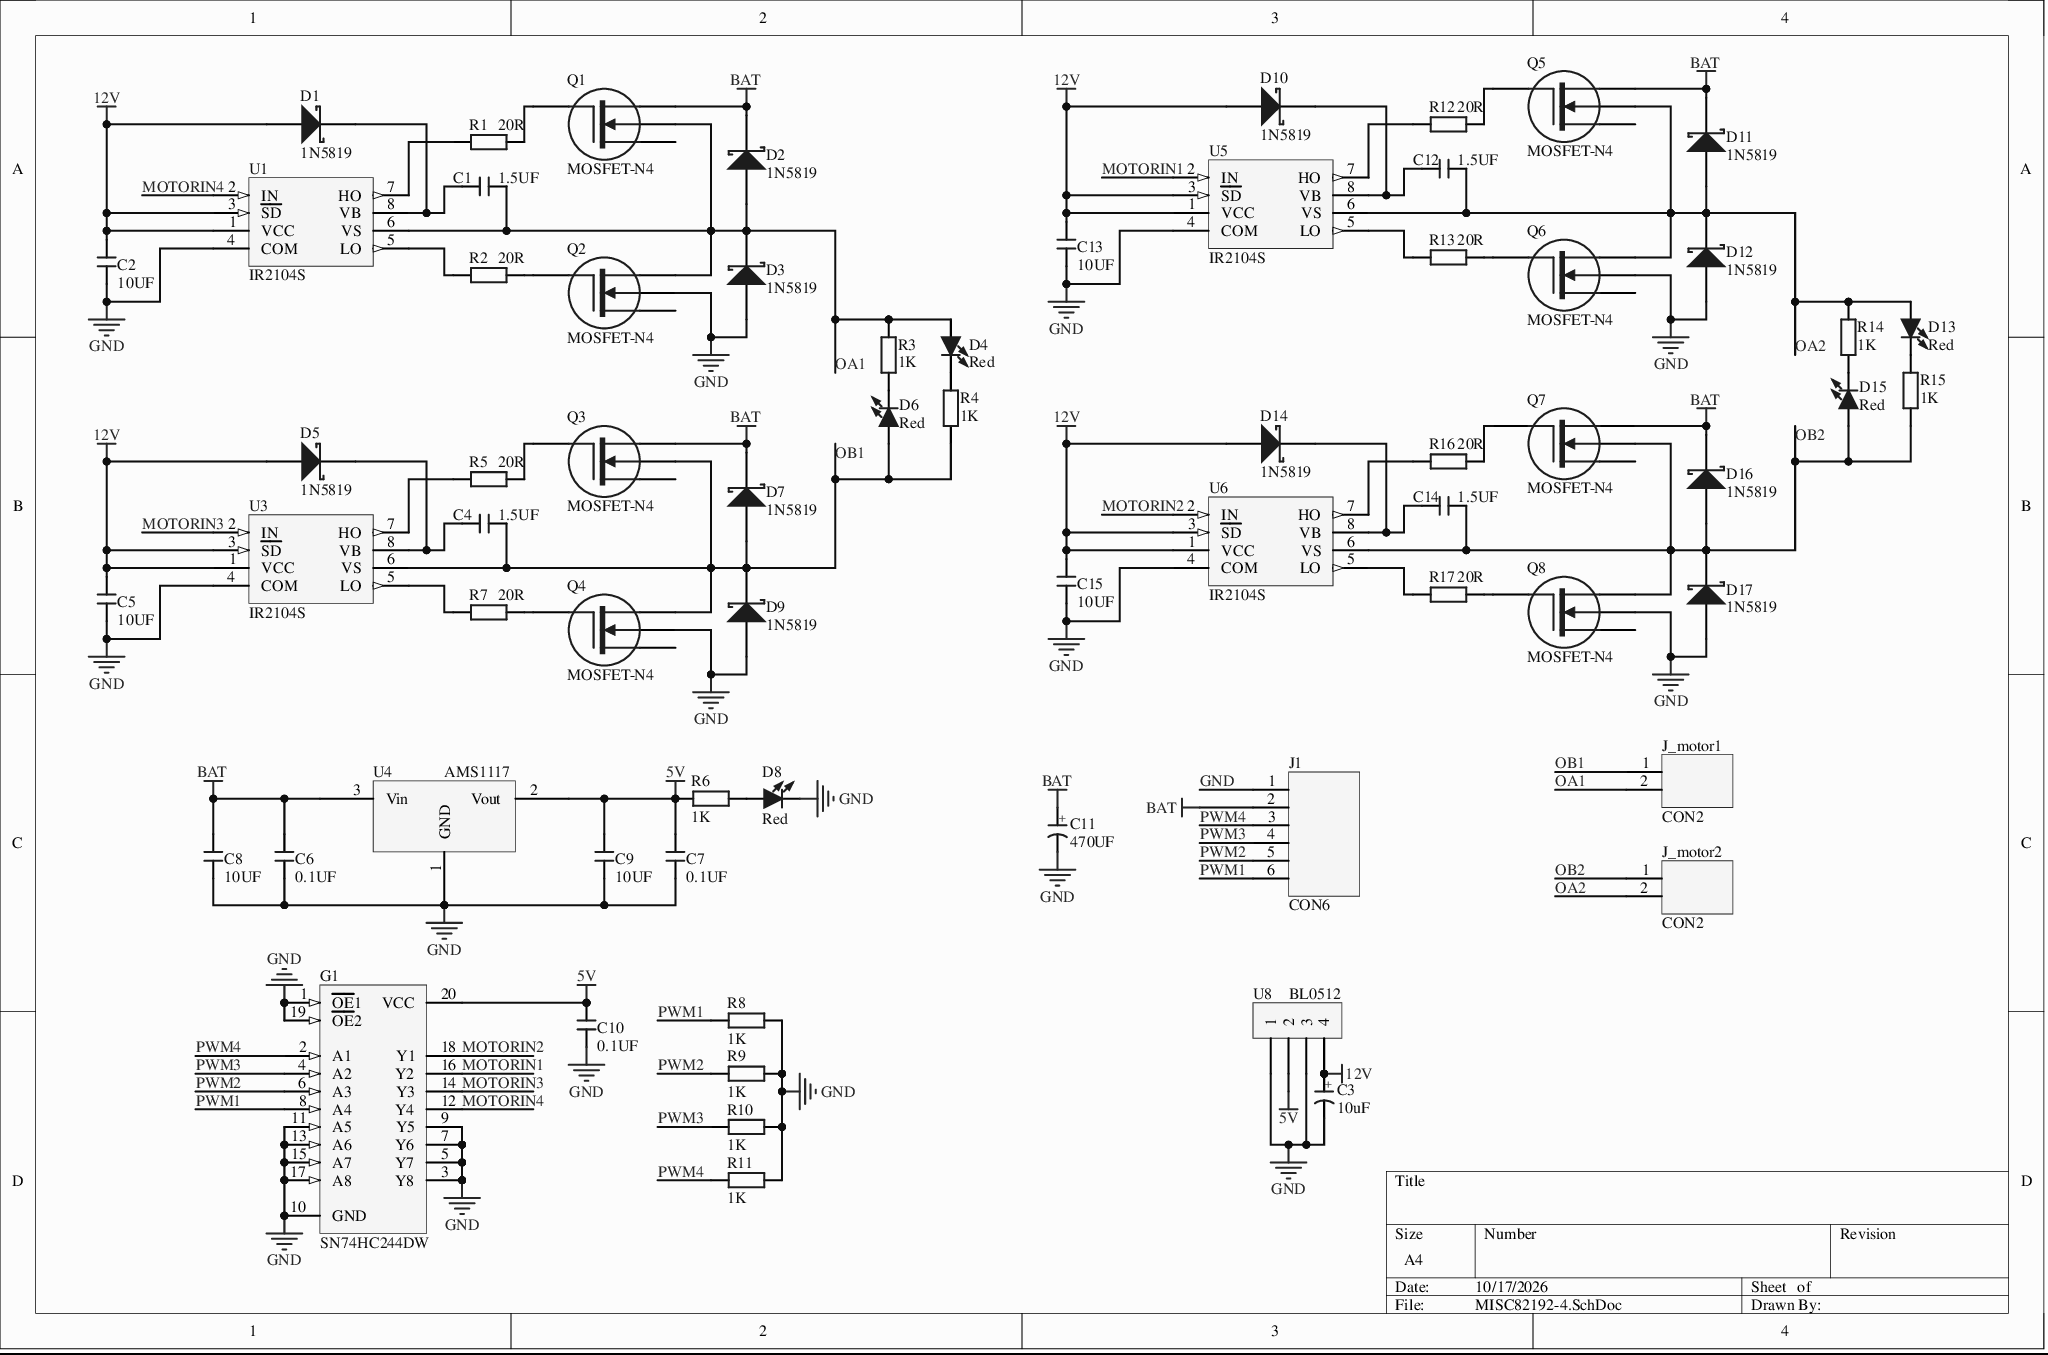
[diagram p0: MISC82192-4.SchDoc]
# Altium project MISC82192-7.PrjPcb
1 sheet, 67 parts. Net scope: global (net labels, ports and power ports of the same name join across sheets).
Board file: MISC82192.PcbDoc

## Sheet MISC82192-4.SchDoc
size A4

### Parts
C1  1.5UF  [C 0805_L]
C2  10UF  [C 0805_L]
C3  10uF  [C 0805_L]
C4  1.5UF  [C 0805_L]
C5  10UF  [C 0805_L]
C6  0.1UF  [C 0805_L]
C7  0.1UF  [C 0805_L]
C8  10UF  [C 0805_L]
C9  10UF  [C 0805_L]
C10  0.1UF  [C 0805_L]
C11  470UF  [CM A(3*5.4)]
C12  1.5UF  [C 0805_L]
C13  10UF  [C 0805_L]
C14  1.5UF  [C 0805_L]
C15  10UF  [C 0805_L]
D1  1N5819  [SOD-323]
D2  1N5819  [SOD-323]
D3  1N5819  [SOD-323]
D4  Red  [LED 0805G]
D5  1N5819  [SOD-323]
D6  Red  [LED 0805G]
D7  1N5819  [SOD-323]
D8  Red  [LED 0805G]
D9  1N5819  [SOD-323]
D10  1N5819  [SOD-323]
D11  1N5819  [SOD-323]
D12  1N5819  [SOD-323]
D13  Red  [LED 0805G]
D14  1N5819  [SOD-323]
D15  Red  [LED 0805G]
D16  1N5819  [SOD-323]
D17  1N5819  [SOD-323]
G1  SN74HC244DW  [DW020]
J1  CON6  [PH2.0-6P]
J_motor1  CON2  [PH2.0-2P]
J_motor2  CON2  [PH2.0-2P]
Q1  MOSFET-N4  [TO252]
Q2  MOSFET-N4  [TO252]
Q3  MOSFET-N4  [TO252]
Q4  MOSFET-N4  [TO252]
Q5  MOSFET-N4  [TO252]
Q6  MOSFET-N4  [TO252]
Q7  MOSFET-N4  [TO252]
Q8  MOSFET-N4  [TO252]
R1  20R  [R 0805_L]
R2  20R  [R 0805_L]
R3  1K  [R 0805_L]
R4  1K  [R 0805_L]
R5  20R  [R 0805_L]
R6  1K  [R 0805_L]
R7  20R  [R 0805_L]
R8  1K  [R 0805_L]
R9  1K  [R 0805_L]
R10  1K  [R 0805_L]
R11  1K  [R 0805_L]
R12  20R  [R 0805_L]
R13  20R  [R 0805_L]
R14  1K  [R 0805_L]
R15  1K  [R 0805_L]
R16  20R  [R 0805_L]
R17  20R  [R 0805_L]
U1  IR2104S  [SOP8]
U3  IR2104S  [SOP8]
U4  AMS1117  [SOT223]
U5  IR2104S  [SOP8]
U6  IR2104S  [SOP8]
U8  BL0512  [Fe-HDR1X4/2.54-S]

### Nets
5V: C7.2 C9.2 C10.2 G1.20(VCC) R6.1 U4.2(Vout) U8.2
12V: C2.2 C3.1(A) C5.2 C13.2 C15.2 D1.1(A) D5.1(A) D10.1(A) D14.1(A) U1.1(VCC) U1.3(~{SD}) U3.1(VCC) U3.3(~{SD}) U5.1(VCC) U5.3(~{SD}) U6.1(VCC) U6.3(~{SD}) U8.4
BAT: C6.2 C8.2 C11.1(A) D2.2(K) D7.2(K) D11.2(K) D16.2(K) J1.2 Q1.4(S) Q3.4(S) Q5.4(S) Q7.4(S) U4.3(Vin)
GND: C2.1 C3.2(K) C5.1 C6.1 C7.1 C8.1 C9.1 C10.1 C11.2(K) C13.1 C15.1 D3.1(A) D8.2(K) D9.1(A) D12.1(A) D17.1(A) G1.1(~{OE}1) G1.3(Y8) G1.5(Y7) G1.7(Y6) G1.9(Y5) G1.10(GND) G1.11(A5) G1.13(A6) G1.15(A7) G1.17(A8) G1.19(~{OE}2) J1.1 Q2.3(U) Q4.3(U) Q6.3(U) Q8.3(U) R8.2 R9.2 R10.2 R11.2 U1.4(COM) U3.4(COM) U4.1(GND) U5.4(COM) U6.4(COM) U8.1 U8.3
MOTORIN1: G1.16(Y2) U5.2(IN)
MOTORIN2: G1.18(Y1) U6.2(IN)
MOTORIN3: G1.14(Y3) U3.2(IN)
MOTORIN4: G1.12(Y4) U1.2(IN)
OA1: C1.1 D2.1(A) D3.2(K) D4.1(A) J_motor1.2 Q1.3(U) Q2.4(S) R3.2 U1.6(VS)
OA2: C12.1 D11.1(A) D12.2(K) D13.1(A) J_motor2.2 Q5.3(U) Q6.4(S) R14.2 U5.6(VS)
OB1: C4.1 D6.1(A) D7.1(A) D9.2(K) J_motor1.1 Q3.3(U) Q4.4(S) R4.2 U3.6(VS)
OB2: C14.1 D15.1(A) D16.1(A) D17.2(K) J_motor2.1 Q7.3(U) Q8.4(S) R15.2 U6.6(VS)
PWM1: G1.8(A4) J1.6 R8.1
PWM2: G1.6(A3) J1.5 R9.1
PWM3: G1.4(A2) J1.4 R10.1
PWM4: G1.2(A1) J1.3 R11.1
NetC1_2: C1.2 D1.2(K) U1.8(VB)
NetC4_2: C4.2 D5.2(K) U3.8(VB)
NetC12_2: C12.2 D10.2(K) U5.8(VB)
NetC14_2: C14.2 D14.2(K) U6.8(VB)
NetD4_2: D4.2(K) R4.1
NetD6_2: D6.2(K) R3.1
NetD8_1: D8.1(A) R6.2
NetD13_2: D13.2(K) R15.1
NetD15_2: D15.2(K) R14.1
NetQ1_1: Q1.1(G) R1.2
NetQ2_1: Q2.1(G) R2.2
NetQ3_1: Q3.1(G) R5.2
NetQ4_1: Q4.1(G) R7.2
NetQ5_1: Q5.1(G) R12.2
NetQ6_1: Q6.1(G) R13.2
NetQ7_1: Q7.1(G) R16.2
NetQ8_1: Q8.1(G) R17.2
NetR1_1: R1.1 U1.7(HO)
NetR2_1: R2.1 U1.5(LO)
NetR5_1: R5.1 U3.7(HO)
NetR7_1: R7.1 U3.5(LO)
NetR12_1: R12.1 U5.7(HO)
NetR13_1: R13.1 U5.5(LO)
NetR16_1: R16.1 U6.7(HO)
NetR17_1: R17.1 U6.5(LO)

Not connected (* = marked no-connect by the designer): Q1 2(D); Q2 2(D); Q3 2(D); Q4 2(D); Q5 2(D); Q6 2(D); Q7 2(D); Q8 2(D)

### Library data of the parts
C1 C2 C4-C10 C12-C15 = C: SMD capacitor; BOM名称: Non-polarized SMD capacitor
C3 = CS_SMD: SMD solid-state capacitor; BOM名称: SMD solid-state capacitor
C11 = CE_SMD: SMD electrolytic capacitor; BOM名称: SMD electrolytic capacitor
D1-D3 D5 D7 D9-D12 D14 D16 D17 = 1N5819: Schottky diode; 属性: 40V/2A; BOM名称: Schottky diode
D4 D6 D8 D13 D15 = LED-SMD: SMD LED; BOM名称: SMD LED
G1 = SN74HC244DW: Octal Buffer and Line Driver with 3-State Outputs; Package Information: Latest Revision: Mar-2000; Code - JEDEC: MS-013; Published: 8-Jun-2000; Revision: 17-Jul-2002: Re-released for DXP Platform.; Datasheet: Latest Revision: May-1997; Package Reference: DW020; Publisher: Altium Limited
J1 = PH2.0-6P
J_motor1 J_motor2 = PH2.0-2P
Q1-Q8 = MOSFET-N4: N-Channel MOSFET, Externally Terminated Substrate; Published: 24-Mar-1999; LatestRevisionDate: 29-May-2009; LatestRevisionNote: IPC-7351 Footprint Added.; PackageVersion: Sep-2000; PackageReference: SOT-343; PackageDescription: 4-Pin SOT-343 Package 1.3 mm Pitch, 2.1 mm Lead Span; Publisher: Altium Limited
R1-R17 = R: SMD resistor; BOM名称: SMD resistor
U1 U3 U5 U6 = IR2104S: High and Low Side Driver; Package Information: Latest Revision: Feb-2001; Code - JEDEC: MS-012-AA; Published: 8-Jun-2000; Revision: 17-Jul-2002: Re-released for DXP Platform.; Datasheet: Latest Revision: PD600461; Package Reference: SO-8; Publisher: Altium Limited
U4 = AMS1117: Three-terminal voltage regulator
U8 = Female HDR1X4